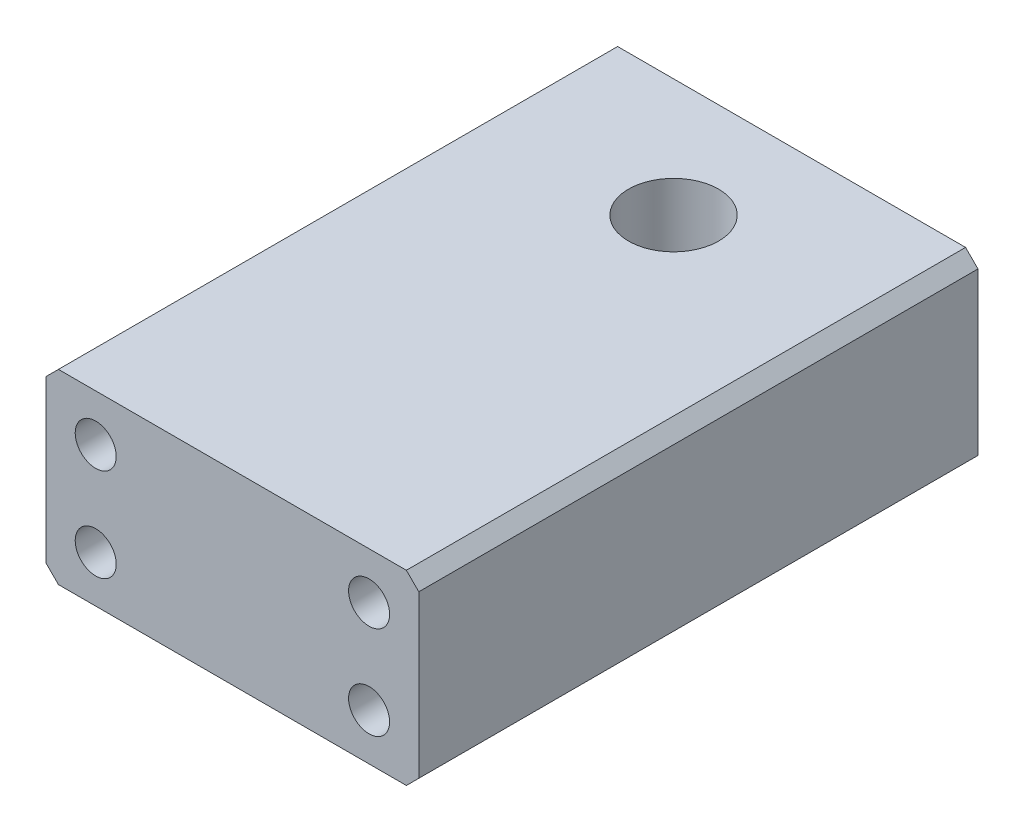
SolidWorks part; units mm, degrees
ref_plane "前视" through (0, 0, 0) normal (0, 0, 1) x (1, 0, 0)
ref_plane "上视" through (0, 0, 0) normal (0, 1, 0) x (1, 0, 0)
ref_plane "右视" through (0, 0, 0) normal (1, 0, 0) x (0, 0, -1)
sketch "草图1" plane through (0, 0, 0) normal (0, 0, 1) x (1, 0, 0)
  line L1 (-30, 15) -> (30, 15)
  line L2 (-30, 15) -> (-30, -15)
  line L3 (-30, -15) -> (30, -15)
  line L4 (30, 15) -> (30, -15)
  line L5 (-30, 15) -> (30, -15) construction
  line L6 (-30, -15) -> (30, 15) construction
  point P0 (0, 0)
  dimension "D1" = 60
  dimension "D2" = 30
extrude "凸台-拉伸1" add sketch "草图1" along normal blind 90
hole_wizard "M16x1.5 螺纹孔1" positions "草图3" profile "草图2" tap size "M16x1.5" standard "GB" end condition through all
sketch "草图3" plane through (0, -15, 0) normal (0, -1, 0) x (-1, 0, 0)
  line L0 (0, -19) -> (0, 0) construction
  point P0 (0, -19)
  dimension "D1" = 19
sketch "草图2" plane through (0, -15, 19) normal (1, 0, 0) x (0, 0, -1)
  line L0 (0, 0) -> (0, 30)
  line L1 (0, 30) -> (7.25, 30)
  line L2 (7.25, 30) -> (7.25, 0)
  line L5 (7.25, 0) -> (0, 0)
  line L11 (0, -6.35) -> (0, 107.95) construction
  dimension "通孔螺纹孔钻头直径" = 14.5
  dimension "通孔螺纹孔钻头深度" = 30
cosmetic thread "孔螺蚊线1" parameters "D2"=16
hole_wizard "M6 六角凹头螺钉的柱形沉头孔1" positions "草图6" profile "草图4" counterbore size "M6" standard "ISO" end condition through all
sketch "草图6" plane through (0, 0, 0) normal (0, 0, -1) x (-1, 0, 0)
  line L0 (0, 0) -> (0, 15) construction
  line L1 (-30, 15) -> (30, 15) construction
  line L3 (22, -7.5) -> (22, 7.5) construction
  line L6 (22, 0) -> (0, 0) construction
  line L8 (30, 15) -> (30, -15) construction
  point P0 (22, -7.5)
  point P2 (22, 7.5)
  point P12 (-22, 7.5)
  point P13 (-22, -7.5)
  dimension "D1" = 15
  dimension "D2" = 8
sketch "草图4" plane through (-22, -7.5, 0) normal (1, 0, 0) x (0, 1, 0)
  line L0 (0, 0) -> (0, 90)
  line L1 (0, 90) -> (3.3, 90)
  line L3 (3.3, 90) -> (3.3, 30)
  line L4 (3.3, 30) -> (5.5, 30)
  line L5 (5.5, 30) -> (5.5, 0)
  line L7 (5.5, 0) -> (0, 0)
  line L11 (0, -6.35) -> (0, 107.95) construction
  dimension "通孔孔直径" = 6.6
  dimension "通孔孔深度" = 90
  dimension "柱形沉头孔直径" = 11
  dimension "柱形沉头孔深度" = 30
chamfer "倒角1" distance 2 angle 45 4 edges at (-30, 15, 45) (-30, -15, 45) (30, 15, 45) (30, -15, 45)
